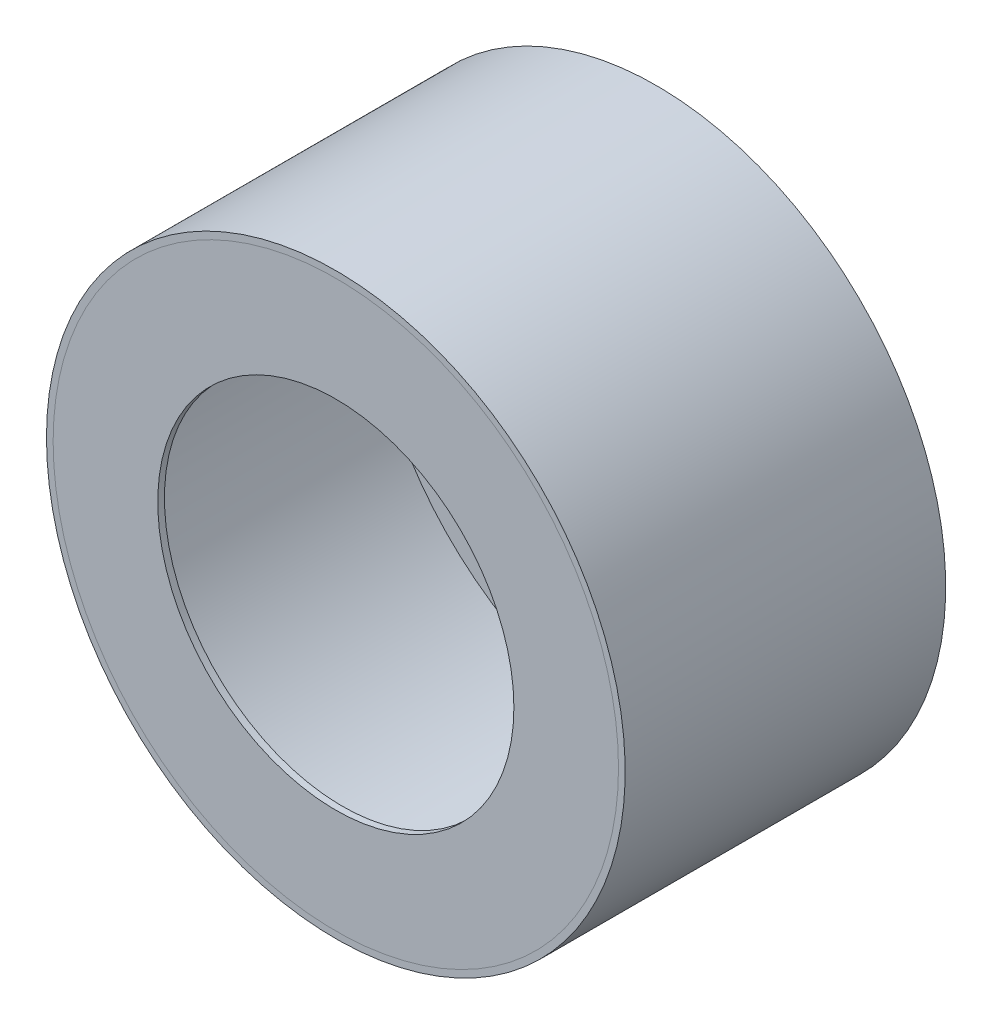
SolidWorks part; units mm, degrees
ref_plane "Front Plane" through (0, 0, 0) normal (0, 0, 1) x (1, 0, 0)
ref_plane "Top Plane" through (0, 0, 0) normal (0, 1, 0) x (1, 0, 0)
ref_plane "Right Plane" through (0, 0, 0) normal (1, 0, 0) x (0, 0, -1)
sketch "Sketch1" plane through (0, 0, 0) normal (0, 0, 1) x (1, 0, 0)
  circle A0 centre (0, 0) radius 325
  dimension "D1" = 650
extrude "Boss-Extrude1" add sketch "Sketch1" along normal blind 360
sketch "Sketch2" plane through (0, 0, 0) normal (0, 0, -1) x (-1, 0, 0)
  circle A0 centre (0, 0) radius 180
  dimension "D1" = 360
extrude "Cut-Extrude1" cut sketch "Sketch2" against normal through all
sketch "Sketch3" plane through (0, 0, 0) normal (0, 0, -1) x (-1, 0, 0)
  circle A0 centre (0, 0) radius 317.5
  dimension "D1" = 635
extrude "Cut-Extrude2" cut sketch "Sketch3" against normal blind 360 from offset 7.5 offset against normal yes
sketch "Sketch4" plane through (0, 0, 0) normal (0, 0, -1) x (-1, 0, 0)
  line L1 (-200, 100) -> (200, 100)
  line L2 (-200, 100) -> (-200, -100)
  line L3 (-200, -100) -> (200, -100)
  line L4 (200, 100) -> (200, -100)
  circle A0 centre (-102.5, 177.5352) radius 5.5
  circle A1 centre (102.5, 177.5352) radius 5.5
  circle A2 centre (102.5, -177.5352) radius 5.5
  circle A3 centre (-102.5, -177.5352) radius 5.5
  dimension "D1" = 11
extrude "Cut-Extrude3" cut sketch "Sketch4" against normal blind 10
sketch "Sketch5" plane through (0, 0, 360) normal (0, 0, 1) x (1, 0, 0)
  circle A0 centre (0, 0) radius 200
  circle A1 centre (0, 0) radius 317.5
  dimension "D1" = 400
extrude "Boss-Extrude2" add sketch "Sketch5" against normal blind 7.5 separate body
